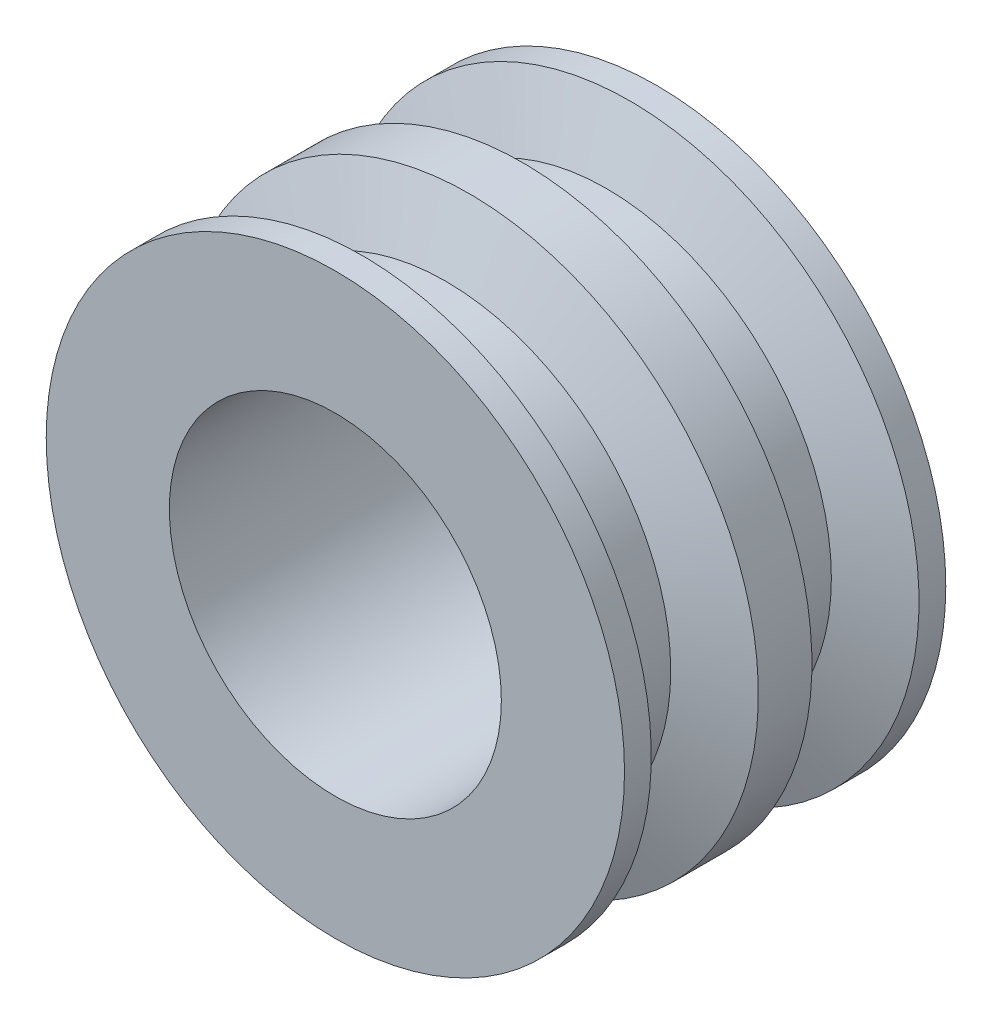
from build123d import *

# Parameters (mm, degrees)
SKETCH1_R           = 27
SKETCH1_R_2         = 15.5
BOSS_EXTRUDE1_DEPTH = 15


with BuildPart() as part:
    # Sketch1 → Boss-Extrude1 (new, symmetric)
    with BuildSketch(Plane.XY):
        Circle(SKETCH1_R)
        Circle(SKETCH1_R_2, mode=Mode.SUBTRACT)
    extrude(amount=BOSS_EXTRUDE1_DEPTH, both=True)

    # Sketch2 → Cut-Revolve1 (revolve, cut)
    with BuildSketch(Plane(origin=(0, 0, 0), x_dir=(1, 0, 0), z_dir=(0, 1, 0))):
        Polygon((-27, -2.5), (-27, -12.5), (-21, -10.316178594), (-21, -4.683821406), align=None)
        Polygon((-27, 2.5), (-21, 4.683821406), (-21, 10.316178594), (-27, 12.5), align=None)
    revolve(axis=Axis((0, 0, -19.218694813), (0, 0, 1)), mode=Mode.SUBTRACT)


solid = part.part
